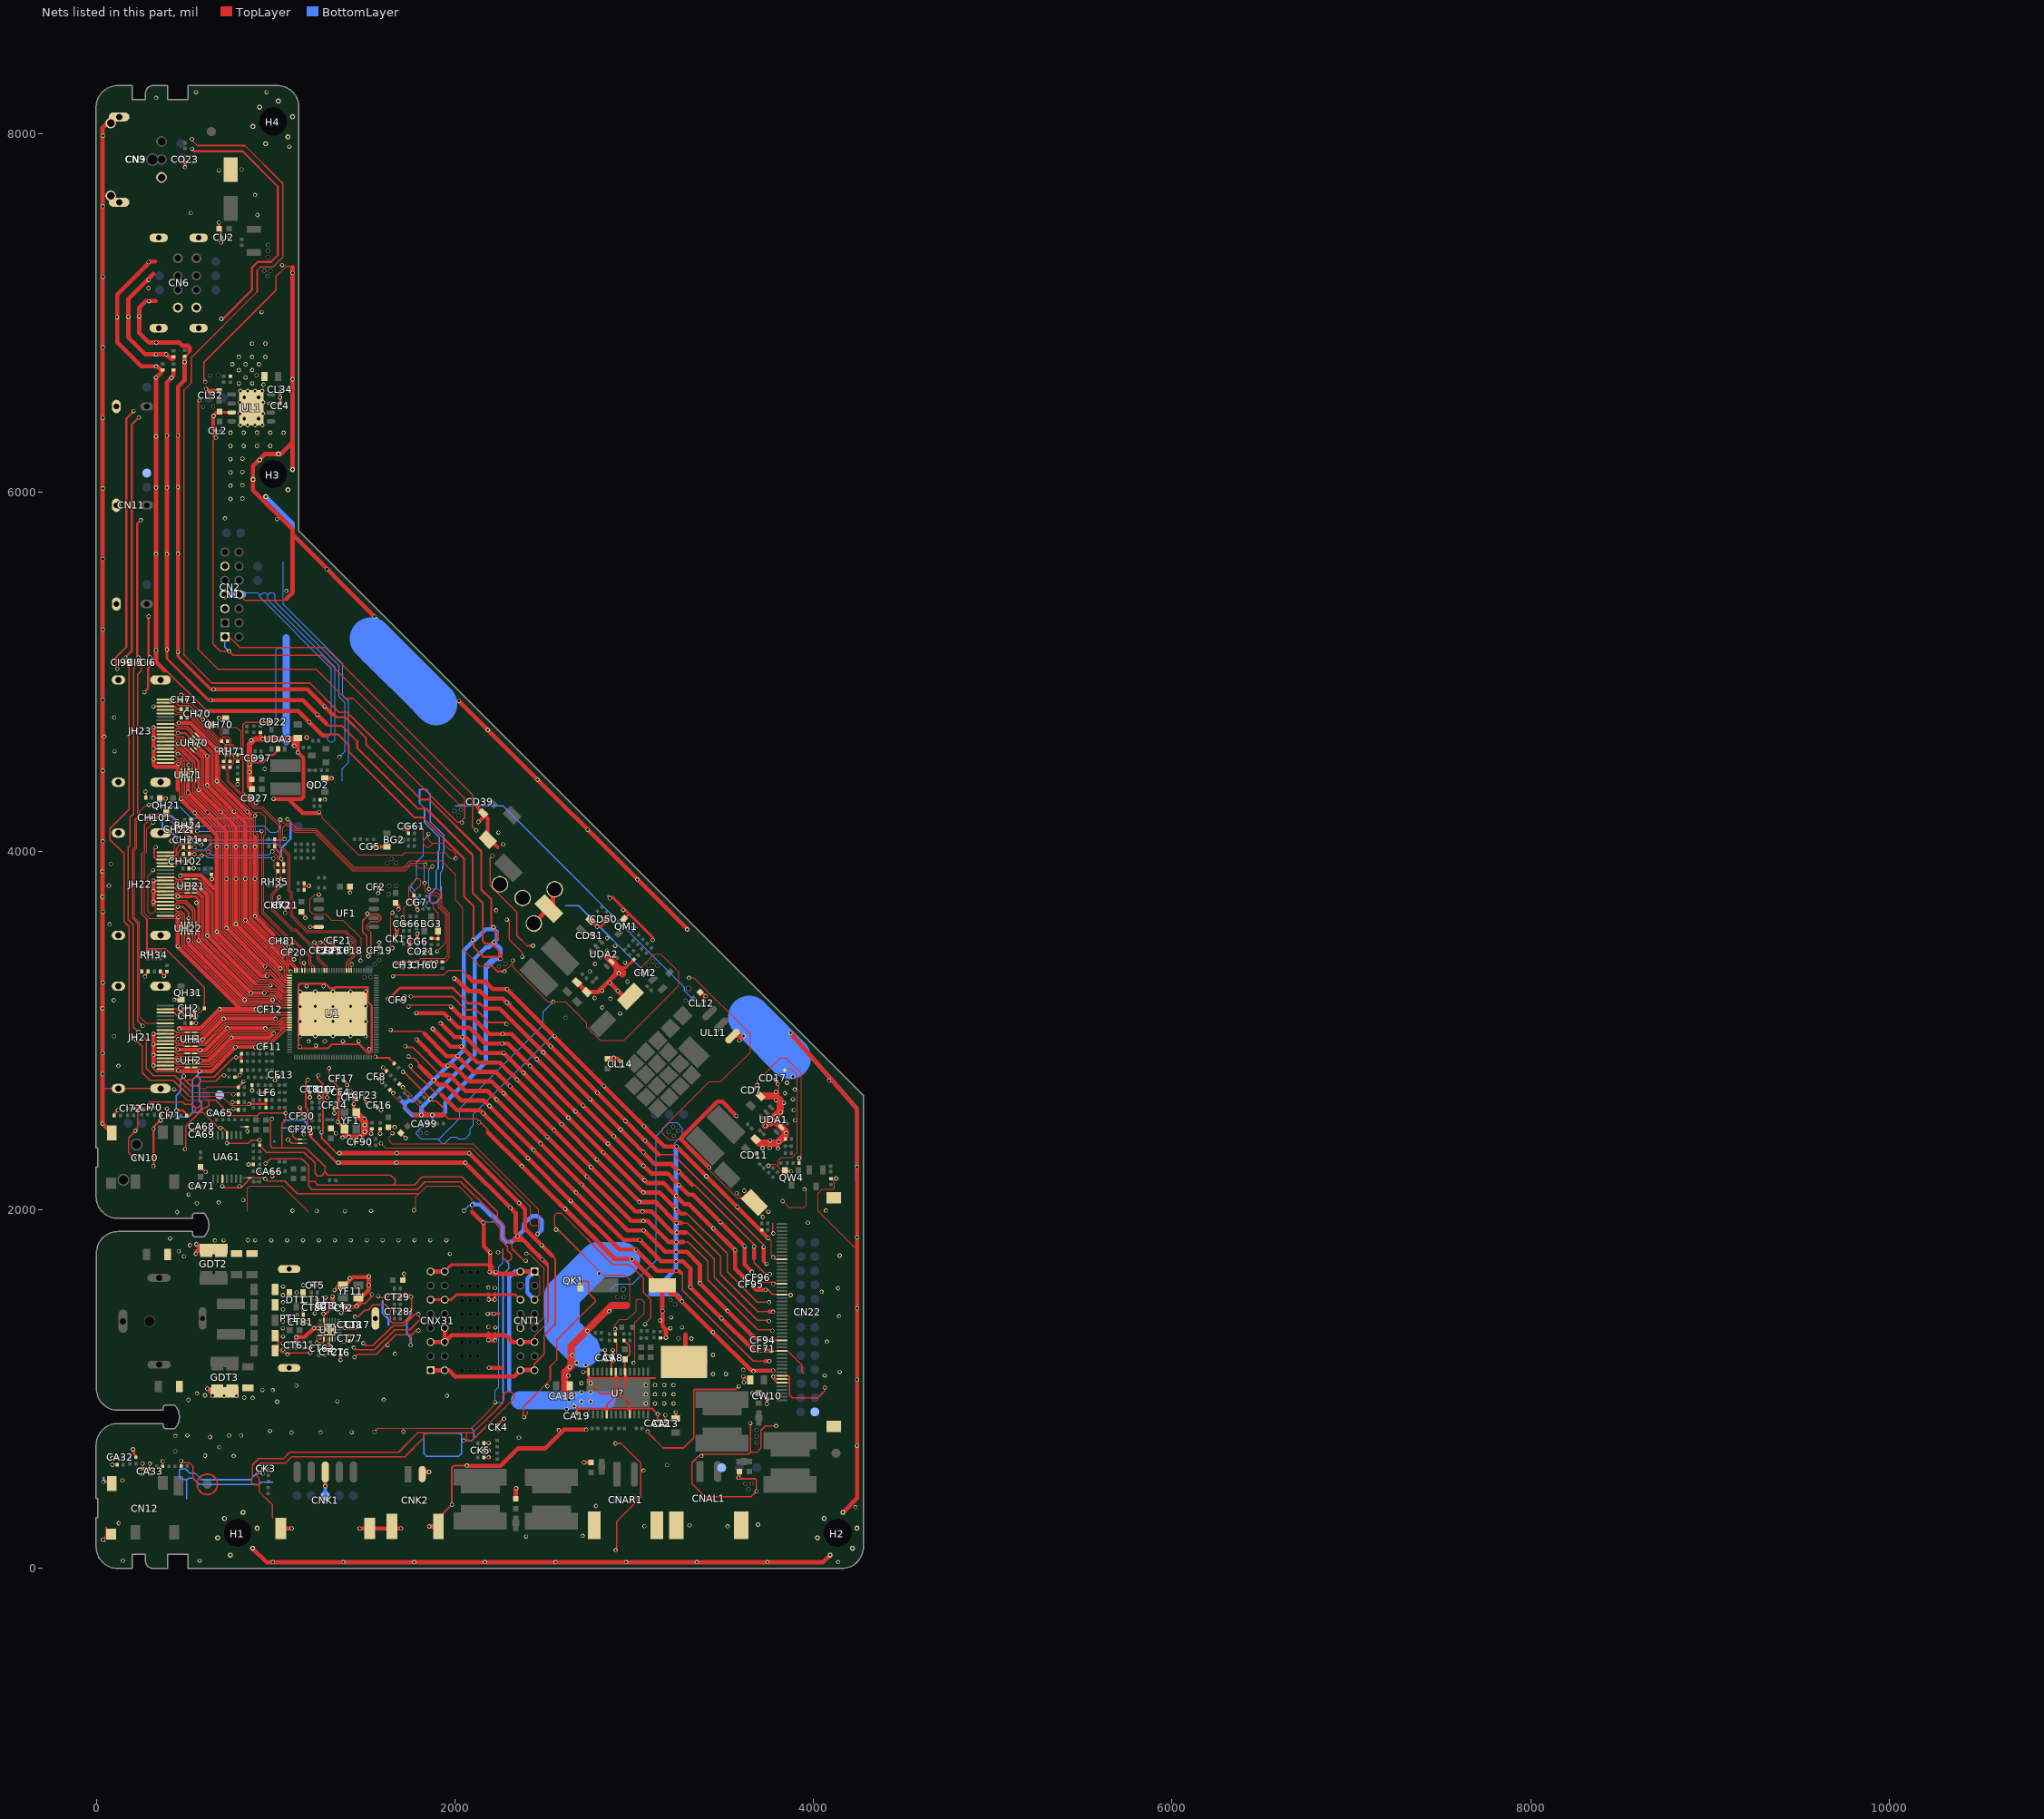
[diagram p0: the nets of this part, all layers, seen from the top]
# Altium PCB MISC105950.PcbDoc (part 10 of 15)
Units mil, origin at the board's own origin, x right, y up, seen from the top; angles counter-clockwise.
Board outline 4280.62 x 8272.76 mil, 2 copper layers (TopLayer, BottomLayer), stack 61.855 mil thick; 541 components, 268 nets, 2324 pads, 1157 vias.

## Via types
v1: diameter 23.62, hole 15.75, TopLayer to BottomLayer, tented both sides, 1087 vias
v2: diameter 23.62, hole 15.75, TopLayer to BottomLayer, 51 vias
v3: diameter 27.56, hole 19.68, TopLayer to BottomLayer, 15 vias
v4: diameter 31.5, hole 19.68, TopLayer to BottomLayer, tented both sides, 4 vias

## Nets (pads, with @x,y where several pads share a name; then routed paths per layer and width w, separated by ;. In a path a pad name is that pad's centre, name@x,y a point inside that pad or via, vN(x,y) a via of type N, cw(c..) or ccw(c..) an arc to the next point about the centre after c; other vN are vias at no path point) (continued)
GND: (continued)
  BottomLayer w15: v1(683,7506.5) v1@683.5,7506 ; v1(1790,3671) v1@1790.5,3671.5 ; v1(2182,1418) v1(2216,1418) ; 2221.5,1529.5 2221.5,1531.5 ; v1@2272.51,831.51 v1(2272.51,832.26) ; v1@2856.5,3742 2856.5,3750.5 ; v1@2893,1333.5 v1(2893.5,1333.5) ; v1@3394,3188.67 v1@3394,3193 ; v1(3739.5,915.5) v1@3740,915
  BottomLayer w20: v1@453.32,2893 v1(453.5,2893) ; GND_KEY.1@1275.9,404.78 v1(1275.9,457.78) ; v1(2615.04,2003.23) v1@2618.53,1999.75
  BottomLayer w24: v1@385,4293 v1(385.5,4292.5) ; v2(556,1806) v2@558,1808 ; H3.6@942.91,5977.37 1093.48,5826.8 1093.48,5711.6 ; 1563.52,5216.53 1563.52,5294.56 ; 1704.5,2600.5 1709.62,2600.5 1719.69,2590.43 ; 1817.55,2659.82 1818.62,2660.88 ; v1(1861.87,2615.5) v1@1859.5,2615.5 ; v1(2094.93,2025) 2104.24,2034.31 ; v1@2097.2,2026.9 2140.7,2026.9 2206.2,1961.4 2206.2,1971.8 2264,1914 2264,1841.81 2285.81,1820 ; 2170.95,3342.45 2225,3396.5 ; 2198,3388 2187,3377 ; v1@2219,1643.5 v1(2226.5,1651) ; 2223.69,1956.93 2223.81,1957.06 ; v1@2289,3155.5 2291.5,3155.5 2303,3144 ; 2300.5,1820 2318.28,1820 2383.5,1885.22 2383.5,1917.69 2428.62,1962.81 ; 2301.5,992.2 2301.5,1063.5 ; 2301.5,1030 2301.5,1063.5 ; CNT1.5@2443.21,1496.63 2403,1536.84 2403,1559.11 2403.12,1559.23 2403.12,1614.02 CNT1.1@2443.21,1654.11 2332.11,1654.11 2301.5,1623.5 2301.5,1063.5 ; 2445,1962.81 2428.62,1962.81 ; v1(2460,1863.5) 2483,1886.5 2483,1940 2460.19,1962.81 ; 2470.29,1952.71 2460.19,1962.81 ; 3034.5,2259.97 v1(3050.97,2243.5) ; 3041.25,2328.18 v1(3051.06,2318.37) ; v1(3235.87,2351.5) 3232,2347.63 3232,1669.51 3089.49,1527 3235.78,1527 3256,1506.78 ; 3861.04,2997.04 4243.09,2561.99 4243.09,2162 ; 1719.69,2590.43 1719.69,2566.57 1758.88,2527.38 1812.43,2527.38 v1(1812.5,2527.31) ; 1719.69,2590.43 1736.57,2607.31 1765.04,2607.31 1818.62,2660.88 ; v1(1812.5,2527.31) 1928.79,2527.31 1945.67,2544.19 1945.67,2595.95 2170.95,2821.23 2170.95,3360.95 2187,3377 ; v1(1812.5,2527.31) 1812.5,2568.5 v1@1859.5,2615.5 ; 1818.62,2660.88 2048.95,2891.21 2048.95,3443.56 2169.69,3564.31 2216.93,3564.31 2233.81,3547.43 2233.81,3508.81 v1(2216.5,3491.5) ; v1@1859.5,2615.5 2109.95,2865.95 2109.95,3400.45 2172.12,3462.62 2187.62,3462.62 v1(2216.5,3491.5) ; 2187,3377 2190.62,3377 2210.12,3396.5 2225,3396.5 ; v1(2216.5,3491.5) 2252.81,3455.19 2252.81,3398.31 2251,3396.5 2225,3396.5 ; 2428.62,1962.81 2460.19,1962.81
  BottomLayer w30: v1(1103,4588) v1@1104,4589
  BottomLayer w40: CN2.5@715.6,5431.32 CN2.6@815.18,5431.32 ; 1057.81,4611 1057.81,5188.69
  BottomLayer w100: 2360.5,935 2845.5,935
  BottomLayer w196.85: 2712.1,1215.9 2597.5,1330.5 2597.5,1522.47 2795.46,1720.43 2933,1720.43
  BottomLayer w236.22: 1530.5,5184.48 1530.5,5183.51 1580.96,5133.05 1581.92,5133.05 1859.43,4855.54 1859.43,4854.58 1894.08,4819.93 1895.04,4819.93 ; 3640.95,3074.03 3640.95,3073.1 3675.59,3038.46 3676.52,3038.46 3868.42,2846.56
  other v1: 983.5,32.5 1377.7,32.5 1771.9,32.5 2166.1,32.5 2560.3,32.5 2954.5,32.5 3348.7,32.5 3742.91,32.5 4137.11,32.5 2396,175.5 2711.5,179.5 3520.5,232.5 3056.5,233 3308,238 3690,242 4233,339 2786,345.5 3051.5,544 3182.7,575.1 4242,681.9 2356.2,726.9 1712,761 2578.5,769.1 1007,928 1342.5,930 1602,939 871,949 824,951 779,960 711,961 1954.5,961 647,962 605,963 560,974 983,992 925,993 4063,1006 3583,1013 2515,1014 1114.5,1018 4242.46,1050.7 4062,1074 4145.5,1094 3665,1098 3608,1106 1065.5,1191.68 1664.5,1194.5 1040,1217.5 1039,1253.5 4074.5,1262.5 2224,1270.5 3246,1281 1040,1291.5 1280.8,1311.3 1318.2,1311.3 1039,1337 2225,1342 3266,1342 2186,1344 1280.8,1348.7 1318.2,1348.7 1039,1376 3144,1381 3205,1398 4142.5,1404.5 1040,1443 4243.09,1449.2 1040,1483 1754,1514 1040,1522.5 1116.5,1536.5 4045,1541 1327,1550 4137,1561 2222,1562 2186,1564 1040,1570 1153,1578 2803.5,1643 488,1739 4145.5,1742.5 1971,1752 2239.5,1761.5 459,1767 520.5,1801 660,1827 707.8,1828 885.4,1828 974.2,1828 1063,1828 1151.8,1828 1240.6,1828 1329.4,1828 1418.2,1828 1507,1828 1595.8,1828 1684.6,1828 1773.4,1828 1862.2,1828 1951,1828 844,1829 4243.09,1844.2 3968.5,1926.5 1385.5,1990 1228,1992 1092.5,1993.5 4069,1994 818,2053 3233.92,2076.47 4243.09,2237.2 3801,2341 3715,2343 3756,2344 3805.06,2378.06 3757,2385 3846.16,2426.97 3759.63,2496.63 3897,2498 3786,2518 3817,2542 3889,2554 247.5,2567 3835,2595 3790,2610 3885,2615 3840,2649 904.5,2653 3790,2656 3895,2670 3852,2707 4086.26,2720.24 3884,2741 32.5,2756.5 122,2801.5 2887,2813 33.5,2873.01 1520.5,2895 1135.25,2908.25 1223,2914.5 1182.5,2938 1273,2938.5 1374,2939 1462,2939 97.5,2966.5 1135.43,2965.89 1501.57,2965.89 1318.97,2967.4 1220.07,2967.86 1416.93,2967.86 234,2990.5 2287.5,3035 1135.43,3048.57 1501.57,3048.57 1318.97,3050.07 1220.07,3050.54 1416.93,3050.54 1965.21,3068.35 2920.5,3093.5 1783.72,3095.81 32.5,3122 2821,3127 1135.43,3131.25 1220.07,3133.22 1318.97,3132.75 1416.93,3133.22 1501.57,3134.2 95.5,3167.5 2866.5,3176 2778,3180 1135.43,3213.92 1318.97,3215.43 1501.57,3215.43 1220.07,3215.89 1416.93,3215.89 2908.14,3219.36 2820,3220 1172,3245.5 1267,3246 2862.62,3264.88 34.5,3266.71 2962.5,3271 2913,3317.5 2751.5,3328.5 2780.5,3370 2949,3377 1101,3395 2811,3406.5 1900,3440.5 2849,3444.5 2892.5,3470.5 2848,3514.5 72.5,3591 512.98,3625 34.5,3660.41 2938,3670.5 557,3711.5 2863.5,3735.5 32.5,3744.5 581.95,3789.33 68.5,3806.5 3016.8,3841.28 724.5,3844.5 883.5,3844.5 32.5,3886.5 80,3928 537.23,3943.5 670.66,4023.5 724.5,4023.5 830.5,4023.5 883.5,4023.5 1573,4024 2267.6,4037.1 34.5,4054.12 2241.8,4103.1 2118,4115.5 2739.53,4118.56 2460.79,4397.3 34.5,4447.82 938,4458.3 512.98,4480 853.65,4483 100,4556.5 863.5,4618.1 1062.1,4624.5 963.2,4626.8 1014.5,4627.4 43.5,4638.86 2181.99,4676.09 1186,4718.5 98,4745.5 1231.5,4761.15 34.5,4841.52 653,4902.5 332,5120 34.5,5235.22 1058.86,5451 1284.78,5573.3 34.5,5628.92 332,5656 393,5656 454,5658.5 1006.04,5852.04 716,5856 34.5,6022.62 332,6313.5 393,6317 454,6317 802.58,6376.63 843.19,6376.63 883.81,6376.63 924.42,6376.63 34.5,6416.32 236.13,6418.51 798.42,6440.87 928.58,6440.87 206.8,6454.6 798.42,6503.13 928.58,6503.13 1023.5,6531 802.58,6567.37 843.19,6567.37 883.81,6567.37 924.42,6567.37 931,6602 1092.85,6632.5 418,6640 331,6642 892,6654 332,6703.76 491,6728 331,6770.76 34.5,6810.02 333,6836.26 696.5,6969 114.66,6978.5 177,6981 238,6983.5 920.5,7006 291.9,7067 290,7141 290.5,7186 34.5,7203.72 1035.5,7269 289.8,7286.7 897,7548 526,7560 34.5,7597.42 884,7660.5 682,7798 808.5,7802.5 1076,7930 34.5,7991.12 332.5,8202 554.5,8233.5 948.2,8233.5
  other v2: 147,41 574.5,41.5 123.5,249.5 144,489 764.5,625 605.5,627 439.5,651 685,673.5 633.5,730.5 439.5,736.5 739.5,739.5 805.5,739.5 506.5,740 1087,755.5 1249,756.5 1423,757.5 966.5,765 512.5,938 553.5,1752.5 410.5,1838 1531.5,1992.5 1770.5,1996 559.5,2035 681,2039.5 513,2083.5
  other v4: 824.13,6412.94 902.87,6412.94 824.13,6531.06 902.87,6531.06
GVDD: CA8.2@2881.84,1155.77 CA8.2@2881.84,1162.66 RA10.1 U?.9 | length 217.7
  TopLayer w10: U?.9@2871.82,1094.5 U?.9@2871.82,1113.5 ; 2871.82,1133.32 U?.9@2871.82,1113.5 ; RA10.1@2892.67,1263.5 2901.69,1254.48 2901.69,1236.5 ; 2901.69,1245 2901.69,1236.5 ; U?.9@2871.82,1113.5 2871.82,1145.75 CA8.2@2881.84,1155.77 2889.06,1155.77 2901.69,1168.4 2901.69,1236.5
HDMI_A_0N_IN_IC: JH23.9 U1.1 UH70.3 UH70.6 | length 1731.4
  TopLayer w7: JH23.9@384.16,4649.61 435.16,4649.61 449,4635.77 482.87,4635.77 500.12,4618.53 ; 500.12,4618.68 500.12,4618.53 ; 560.22,4558.42 560.22,4563.65 UH70.6@547.26,4576.61 UH70.3@518.3,4605.56 505.34,4618.53 500.12,4618.53 ; 561.28,4557.36 596.98,4521.66 596.98,4359.49 810,4146.48 810,3606.05 967.27,3448.77 ; 938.02,3478.02 967.27,3448.77 ; U1.1@1076.34,3305.46 1063.18,3305.46 1058,3310.64 1058,3358.05 967.27,3448.77
HDMI_A_0P_IN_IC: JH23.7 U1.2 UH70.4 UH70.5 | length 1761.3
  TopLayer w7: JH23.7@384.16,4610.24 432.97,4610.24 446.5,4623.77 ; 446.61,4623.66 478.01,4623.66 490.57,4611.1 490.57,4605.46 UH70.4@504.38,4591.64 UH70.5@533.34,4562.69 547.15,4548.88 552.8,4548.88 558.81,4542.87 584.98,4516.69 584.98,4354.52 798,4141.51 798,3601.08 1023.04,3376.04 ; 974.08,3425 1023.04,3376.04 ; U1.2@1076.34,3291.68 1059.99,3291.68 1046,3305.67 1046,3353.08 1023.04,3376.04
HDMI_A_1N_IN_IC: JH23.6 U1.3 UH71.1 UH71.8 | length 1656.7
  TopLayer w7: JH23.6@384.16,4590.55 435.16,4590.55 449,4576.72 470.66,4576.72 548.66,4498.71 548.66,4466.33 552.35,4462.64 UH71.1@552.35,4444.3 552.35,4385.02 548.66,4381.33 548.66,4332.87 757,4124.52 757,3584.09 1034,3307.09 1034,3300.23 1056.33,3277.9 U1.3@1076.34,3277.9
HDMI_A_1P_IN_IC: JH23.4 U1.4 UH71.2 UH71.7 | length 1666.6
  TopLayer w7: JH23.4@384.16,4551.18 432.97,4551.18 446.5,4564.72 465.68,4564.72 536.66,4493.74 536.66,4467.83 532.67,4463.84 532.67,4383.82 536.66,4379.83 536.66,4351 ; 536.66,4341.98 536.66,4351 ; U1.4@1076.34,3264.12 1053.14,3264.12 1022,3295.26 1022,3302.12 745,3579.12 745,4119.55 536.66,4327.9 536.66,4351
HDMI_A_2N_IN_IC: JH23.3 U1.5 UH71.3 UH71.6 | length 1647.4
  TopLayer w7: JH23.3@384.16,4531.5 435.16,4531.5 449,4517.66 470.56,4517.66 489.6,4498.62 489.6,4467.83 ; 489.6,4466.33 493.3,4462.64 493.3,4385.02 489.6,4381.33 489.6,4316.97 704,4102.57 704,3562.14 930.52,3335.62 964.67,3335.62 1049.95,3250.34 U1.5@1076.34,3250.34
HDMI_A_2P_IN_IC: JH23.1 U1.6 UH71.4 UH71.5 | length 1649.8
  TopLayer w7: JH23.1@384.16,4492.13 432.97,4492.13 446.5,4505.66 465.59,4505.66 477.6,4493.65 477.6,4467.83 473.61,4463.84 UH71.4@473.61,4444.3 473.61,4383.82 477.6,4379.83 477.6,4312 692,4097.6 692,3557.17 925.55,3323.62 959.7,3323.62 1046.76,3236.56 U1.6@1076.34,3236.56
HDMI_A_5V: CH70.1 JH23.18 RH70.2 RH71.2 RH71.4 RH71.6 RH74.2 | length 1006.3
  TopLayer w5: 744.5,4589.98 747.59,4593.07 747.59,4593.16 747.59,4624.95 733.2,4639.34 701.62,4639.34 692.81,4648.15 692.81,4685.85 697.21,4690.25 781.25,4690.25 805.15,4666.35 805.15,4597.42 805.15,4517.39 RH74.2@787.75,4499.99
  TopLayer w8: JH23.18@384.16,4826.77 443.23,4826.77 457.67,4812.33 517.82,4812.33 546,4784.15 546,4749.26 564.63,4730.63 ; 574.57,4720.69 564.63,4730.63 ; 651.88,4643.38 645.88,4649.38 ; RH70.2@697.3,4612 683.26,4612 645.88,4649.38 ; RH70.2@697.54,4611.77 716.15,4593.16 ; RH71.2@720.88,4573.5 720.88,4588.43 716.15,4593.16 ; 741.32,4593.16 716.15,4593.16 ; RH71.4@744.5,4573.5 744.5,4589.98 ; 744.5,4593.16 747.59,4593.16 757.84,4593.16 764.19,4586.81 RH71.6@764.19,4573.5 ; 564.63,4730.63 645.88,4649.38
HDMI_A_CKN_IN_IC: JH23.12 U1.127 UH70.1 UH70.8 | length 1746.2
  TopLayer w7: JH23.12@384.16,4708.66 435.16,4708.66 449,4694.83 507.34,4694.83 541.88,4660.29 ; 541.88,4660.44 541.88,4660.29 ; U1.127@1118.7,3334.04 1118.7,3348.26 1074.21,3392.75 1074.21,3416.79 863,3628 863,4168.43 649.98,4381.45 649.98,4552.18 601.98,4600.18 601.98,4605.41 UH70.8@589.01,4618.37 UH70.1@560.06,4647.32 547.1,4660.29 541.88,4660.29
HDMI_A_CKP_IN_IC: JH23.10 U1.128 UH70.2 UH70.7 | length 1725.5
  TopLayer w7: JH23.10@384.16,4669.29 432.97,4669.29 446.5,4682.83 446.61,4682.72 502.47,4682.72 532.33,4652.86 532.33,4647.22 UH70.2@546.14,4633.4 UH70.7@575.1,4604.45 588.91,4590.64 594.56,4590.64 637.98,4547.21 637.98,4376.48 851,4163.46 851,3623.03 1062.21,3411.82 1062.21,3387.78 1104.92,3345.07 U1.128@1104.92,3334.04
HDMI_A_HPD_OUT: CH71.1 JH23.19 QH70.C RH70.1 | length 476.1
  TopLayer w5: JH23.19@384.16,4846.46 CH71.1@468.81,4846.46 ; CH71.1@471.77,4840.23 471.77,4828.73 475.67,4824.83 529.98,4824.83 623.65,4731.15 623.65,4718.16 636.81,4705 QH70.C@641.97,4705 641.97,4669.55 682.18,4629.34 713.89,4629.34 RH70.1@731.23,4612 ; CH71.1@471.77,4843.5 CH71.1@473.4,4841.86
HDMI_A_HPD_OUT_IC: RH71.5 RH71.7 U1.120 | length 1571.8
  TopLayer w5: RH71.5@764.19,4538.07 766.5,4535.75 766.5,4516.5 ; RH71.7@787.81,4538.07 787.81,4520.81 783.5,4516.5 766.5,4516.5 ; U1.120@1215.15,3334.04 1215.15,3353.63 1195.66,3373.13 1195.66,3411.08 1090.27,3516.47 1073.53,3516.47 933,3656.99 933,4086 941.81,4094.81 941.81,4187.66 912.48,4216.98 871.02,4216.98 689.98,4398.01 689.98,4477.06 695.55,4482.63 756.7,4482.63 766.5,4492.42 766.5,4516.5
HDMI_A_SCL_IN: DH71.K JH23.15 RH71.1 RH72.1 | length 491.3
  TopLayer w5: JH23.15@384.16,4767.72 432.78,4767.72 437.67,4762.83 487.9,4762.83 DH71.K@506.23,4744.5 520.35,4744.5 693.54,4571.31 693.54,4543.96 699.43,4538.07 RH71.1@720.88,4538.07 720.88,4512.11 RH72.1@708.5,4499.73
HDMI_A_SCL_IN_IC: RH72.2 U1.107 | length 1616.3
  TopLayer w5: RH72.2@708.5,4466.27 708.5,4466 728.81,4445.69 728.81,4387.47 779.42,4336.86 ; 767,4349.28 779.42,4336.86 ; U1.107@1394.29,3334.04 1394.19,3334.13 1394.19,3381.25 1435.31,3422.37 1435.31,3496 1385,3546.31 1173.56,3546.31 1121.24,3598.64 1121.02,3598.64 1081,3638.66 1081,3766 1070.36,3776.64 1070.36,3974.64 1019.86,4025.14 1019.86,4138.1 933.96,4224 933.75,4224 920.77,4236.98 879.3,4236.98 779.42,4336.86
HDMI_A_SDA_IO: DH72.K JH23.16 RH71.3 RH73.1 | length 527.9
  TopLayer w5: JH23.16@384.16,4787.4 433.6,4787.4 448.17,4772.83 487.56,4772.83 DH72.K@506.23,4791.5 527.42,4770.31 527.42,4751.57 703.54,4575.46 703.54,4560.55 708.68,4555.41 733.83,4555.41 RH71.3@744.5,4544.74 ; RH73.1@744.5,4506.23 RH71.3@744.5,4538.07
HDMI_A_SDA_IO_IC: RH73.2 U1.106 | length 1608.4
  TopLayer w5: 738.81,4392.7 738.81,4391.61 ; RH73.2@744.5,4466.27 738.81,4460.58 738.81,4391.61 ; 1257.5,3556.31 1265.5,3556.31 ; U1.106@1406.12,3329 U1.106@1406.12,3334.04 ; U1.106@1408.07,3334.04 1408.07,3356.52 1404.19,3360.39 1404.19,3377.11 1445.31,3418.23 1445.31,3500.14 1389.14,3556.31 1265.5,3556.31 ; 738.81,4391.61 883.44,4246.98 924.91,4246.98 937.89,4234 938.1,4234 1029.86,4142.24 1029.86,4029.28 1080.36,3978.78 1080.36,3780.78 1091,3770.14 1091,3642.8 1125.16,3608.64 1125.38,3608.64 1177.7,3556.31 1265.5,3556.31
HDMI_ARC_OUT: CH81.1 DH81.K JH21.14 | length 2780.3
  TopLayer w5: v1@287,4253 272.31,4253 240.31,4221 240.31,4182 225,4166.69 225,4016.26 211.5,4002.76 211.5,3630.31 239.5,3602.31 239.5,3341.77 DH81.K@252.77,3328.5 239.5,3315.23 239.5,3074.5 274.63,3039.37 JH21.14@384.16,3039.37 ; v1@886,4195.5 886,4104.08 903,4087.08 903,3644.57 1025.17,3522.4 CH81.1@1025.17,3508.83
  BottomLayer w5: v1(291.5,4257.5) 300.81,4266.81 339.5,4266.81 359.95,4246.36 465.09,4246.36 526.95,4184.5 871,4184.5 v1(884,4197.5)
HDMI_ARC_OUT_IC: CH81.2@1043.96,3490.04 CH81.2@1048.83,3485.17 U1.125 | length 210.2
  TopLayer w5: CH81.2@1048.83,3485.17 1049.98,3486.31 1078,3486.31 1137.31,3427 1137.31,3369.24 1146.26,3360.3 U1.125@1146.26,3334.04
HDMI_B_0N_IN_IC: JH22.9 U1.9 UH21.3 UH21.6 | length 1076.2
  TopLayer w7: JH22.9@384.16,3795.28 435.16,3795.28 449,3781.44 484.39,3781.44 484.5,3781.33 488.19,3785.02 UH21.3@506.53,3785.02 UH21.6@547.47,3785.02 557.27,3785.02 597.16,3745.13 597.16,3519.08 874.42,3241.81 950.12,3241.81 961.93,3230 1002.41,3230 1037.19,3195.22 U1.9@1076.34,3195.22
HDMI_B_0P_IN_IC: JH22.7 U1.10 UH21.4 UH21.5 | length 1073.6
  TopLayer w7: JH22.7@384.16,3755.91 432.97,3755.91 446.5,3769.44 ; 446.61,3769.33 483,3769.33 486.99,3765.34 UH21.4@506.53,3765.34 UH21.5@547.47,3765.34 559.98,3765.34 585.16,3740.16 585.16,3514.11 869.45,3229.81 945.15,3229.81 956.96,3218 997.44,3218 1034,3181.44 U1.10@1076.34,3181.44
HDMI_B_1N_IN_IC: JH22.6 U1.11 UH22.1 UH22.8 | length 1082.8
  TopLayer w7: JH22.6@384.16,3736.22 435.16,3736.22 449,3722.39 ; 484.5,3722.39 449,3722.39 ; U1.11@1076.34,3167.66 1030.81,3167.66 995.47,3203 969.46,3203 955.46,3189 852.28,3189 838.28,3203 548.66,3492.62 548.66,3527 552.35,3530.69 UH22.8@552.35,3549.03 UH22.1@552.35,3589.97 552.35,3608.31 548.66,3612 548.66,3671.84 498.11,3722.39 449,3722.39
HDMI_B_1P_IN_IC: JH22.4 U1.12 UH22.2 UH22.7 | length 1094.6
  TopLayer w7: JH22.4@384.16,3696.85 432.97,3696.85 446.5,3710.39 466,3710.39 ; 483,3710.39 466,3710.39 ; 648.5,3375.81 669.3,3355.02 ; U1.12@1076.34,3153.89 1027.61,3153.89 990.5,3191 974.43,3191 960.43,3177 847.31,3177 669.3,3355.02 ; 466,3710.39 493.14,3710.39 536.66,3666.87 536.66,3613.5 532.67,3609.51 UH22.2@532.67,3589.97 UH22.7@532.67,3549.03 532.67,3529.49 536.66,3525.5 536.66,3487.65 669.3,3355.02
HDMI_B_2N_IN_IC: JH22.3 U1.13 UH22.3 UH22.6 | length 1053.4
  TopLayer w7: JH22.3@384.16,3677.17 435.16,3677.17 449,3663.33 472.47,3663.33 489.6,3646.2 489.6,3613.5 ; 489.6,3612 493.3,3608.31 UH22.3@493.3,3589.97 UH22.6@493.3,3549.03 493.3,3530.69 489.6,3527 489.6,3476.73 633.29,3333.04 ; 607.5,3358.83 633.29,3333.04 ; U1.13@1076.34,3140.11 1056.28,3140.11 1054.5,3138.33 1018.77,3138.33 1007.1,3150 816.33,3150 633.29,3333.04
HDMI_B_2P_IN_IC: JH22.1 U1.14 UH22.4 UH22.5 | length 1046.2
  TopLayer w7: JH22.1@384.16,3637.8 432.97,3637.8 446.5,3651.33 467.5,3651.33 477.6,3641.23 477.6,3613.5 473.61,3609.51 UH22.4@473.61,3589.97 UH22.5@473.61,3549.03 473.61,3529.49 477.6,3525.5 477.6,3471.75 615.56,3333.79 ; 595.5,3353.86 615.56,3333.79 ; U1.14@1076.34,3126.33 1013.8,3126.33 1002.13,3138 811.36,3138 615.56,3333.79
HDMI_B_5V: CH21.1 JH22.18 RH1.2 RH23.2 RH24.2 RH24.4 RH24.6 | length 2572.1
  TopLayer w5: v1(1049.17,4066.69) 1039.86,4076 1039.86,4131.81 1051.17,4143.12 1067.17,4143.12 1104.79,4105.5 1213.28,4105.5 1427.78,3891 1722.49,3891 1751.3,3919.81 1782.9,3919.81 1797.03,3905.69 v1@1873.19,3905.69 ; v1(1854.5,3788) 1905.5,3788 1926.5,3767 1926.5,3694.14 1968.31,3652.33 1968.31,3404.54 1944.5,3380.73 RH1.2@1929,3380.73
  TopLayer w8: JH22.18@384.16,3972.44 440.18,3972.44 445.74,3978.01 445.74,4014.93 473.37,4042.55 512.55,4042.55 517.07,4047.07 CH21.1@517.07,4056.98 ; 470.84,4132.5 RH24.4@491.5,4132.5 ; 491.5,4097.34 CH21.1@517.07,4071.77 ; RH24.2@491.5,4108.88 472.12,4108.88 468.34,4112.66 468.34,4146.34 474.19,4152.18 RH24.6@491.5,4152.18 ; CH21.1@517.07,4067.93 CH21.1@517.07,4062.1 517.68,4061.5 v1(543.74,4061.5) RH23.2@573.77,4061.5
  BottomLayer w5: v1(543.74,4061.5) v1@1043.98,4061.5 ; v1(1854.5,3788) 1854.5,3894.5 v1(1874,3914)
HDMI_B_CKN_IN_IC: JH22.12 U1.7 UH21.1 UH21.8 | length 1089.3
  TopLayer w7: JH22.12@384.16,3854.33 435.16,3854.33 449,3840.5 484.39,3840.5 484.5,3840.39 488.19,3844.08 UH21.1@506.53,3844.08 UH21.8@547.47,3844.08 565.81,3844.08 573.49,3836.39 580.85,3836.39 650.16,3767.09 650.16,3541.03 908.57,3282.62 983.73,3282.62 1043.57,3222.78 U1.7@1076.34,3222.78
HDMI_B_CKP_IN_IC: JH22.10 U1.8 UH21.2 UH21.7 | length 1086.8
  TopLayer w7: JH22.10@384.16,3814.96 432.97,3814.96 446.5,3828.5 446.61,3828.39 483,3828.39 486.99,3824.39 UH21.2@506.53,3824.39 UH21.7@547.47,3824.39 575.88,3824.39 638.16,3762.12 638.16,3536.06 903.6,3270.62 978.76,3270.62 1040.38,3209 U1.8@1076.34,3209
HDMI_B_HPD_OUT: CH22.1 JH22.19 QH21.C RH23.1 | length 573.8
  TopLayer w5: JH22.19@384.16,3992.13 426.87,3992.13 434.24,3999.5 434.24,4010.5 ; QH21.C@388.5,4214.47 430.19,4172.78 430.19,4120.31 CH22.1@445.73,4104.77 ; v1(417,4056) 430.74,4056 ; 434.24,4035 434.24,4010.5 ; 434.24,4040.74 434.24,4056 ; CH22.1@449.5,4104.77 434.24,4089.51 434.24,4056 ; v1(585.23,4033.85) 579.58,4033.85 RH23.1@607.23,4061.5 ; 434.24,4010.5 434.24,4056
  BottomLayer w5: v1(417,4056) 431.95,4041.05 567.05,4041.05 574.26,4033.85 v1(585.23,4033.85)
HDMI_B_HPD_OUT_IC: RH24.5 RH24.7 U1.121 | length 1432.1
  TopLayer w5: RH24.5@526.93,4152.18 542.96,4152.18 ; RH24.7@526.93,4175.81 538.69,4175.81 544.28,4170.22 544.28,4130.72 v1@561,4114 ; v1@918.12,4110.88 v1(920.65,4110.88) 923,4108.53 923,3938 ; 923,4006.5 923,3938 ; U1.121@1201.37,3334.04 1201.37,3353.27 1186.66,3367.99 1186.66,3405.94 1086.28,3506.31 1069.54,3506.31 923,3652.85 923,3938
  BottomLayer w5: v1@561.38,4110.88 v1(920.65,4110.88)
  other v1: 561,4110.5
HDMI_B_SCL_IN: DH22.K DH75.K JH22.15 RH24.1 RH35.3 | length 1060.9
  TopLayer w5: JH22.15@384.16,3913.39 439.24,3913.39 453.5,3927.64 453.5,3952.27 DH22.K@485.33,3984.1 506.62,3962.81 557.5,3962.81 569.69,3975 v1(585.23,3975) ; RH24.1@526.93,4108.88 545,4090.81 628.08,4090.81 641.16,4077.73 641.16,3988.16 630.19,3977.19 592.64,3977.19 v1@585.23,3969.77 ; v1@991.81,3953 991.81,3906.23 DH75.K@1010.54,3887.5 1003.84,3880.81 RH35.3@1003.84,3844.22
  BottomLayer w5: v1@585.23,3969.77 v1@586.5,3971.05 ; v1@586.5,3974 607.81,3974 619.5,3962.31 v1@982.5,3962.31
  other v1: 986.07,3958.74
HDMI_B_SCL_IN_IC: RH35.4 U1.116 | length 620.5
  TopLayer w5: RH35.4@1003.84,3808.78 1003.84,3788.94 973,3758.09 973,3673.56 1090.1,3556.47 1106.84,3556.47 1231.66,3431.65 1231.66,3393.7 1270.27,3355.08 U1.116@1270.27,3334.04
HDMI_B_SDA_IO: DH23.K DH76.K JH22.16 RH24.3 RH35.1 | length 1107.4
  TopLayer w5: JH22.16@384.16,3933.07 438.57,3933.07 442.46,3936.96 442.46,3957.72 457.24,3972.5 457.24,3994.01 483.11,4019.89 500.57,4002.43 v1@615.57,4002.43 ; RH24.3@526.93,4132.5 520.26,4132.5 509.59,4121.83 509.59,4095.52 524.29,4080.81 623.93,4080.81 631.16,4073.59 631.16,4006.16 v1(621.5,3996.5) ; v1(981,3998.5) 1010.54,3968.96 DH76.K@1010.54,3926 1027.46,3909.07 RH35.1@1027.46,3844.22
  BottomLayer w5: v1(621.5,3996.5) 638.81,3979.19 961.69,3979.19 v1(981,3998.5)
HDMI_B_SDA_IO_IC: RH35.2 U1.115 | length 627.7
  TopLayer w5: RH35.2@1027.46,3808.78 1027.46,3798.42 983,3753.95 983,3677.71 1094.24,3566.47 1110.98,3566.47 1240.66,3436.79 1240.66,3398.84 1284.05,3355.44 U1.115@1284.05,3334.04
HDMI_C_0N_IN_IC: JH21.9 U1.18 UH1.3 UH1.6 | length 760.8
  TopLayer w7: JH21.9@384.16,2940.95 435.16,2940.95 449,2927.11 484.39,2927.11 484.5,2927 488.19,2930.69 UH1.3@506.53,2930.69 UH1.6@547.47,2930.69 565.81,2930.69 569.5,2927 599.94,2927 716.94,3044 1010.12,3044 1035.55,3069.43 1060.75,3069.43 1062.53,3071.21 U1.18@1076.34,3071.21
HDMI_C_0P_IN_IC: JH21.7 U1.19 UH1.4 UH1.5 | length 760
  TopLayer w7: JH21.7@384.16,2901.58 432.97,2901.58 446.5,2915.11 ; 446.61,2915 483,2915 486.99,2911.01 UH1.4@506.53,2911.01 UH1.5@547.47,2911.01 567.01,2911.01 571,2915 604.92,2915 721.92,3032 1015.09,3032 1040.52,3057.43 U1.19@1076.34,3057.43
HDMI_C_1N_IN_IC: JH21.6 U1.20 UH2.1 UH2.8 | length 784.3
  TopLayer w7: JH21.6@384.16,2881.89 435.16,2881.89 449,2868.06 484.5,2868.06 488.19,2871.75 UH2.1@506.53,2871.75 UH2.8@547.47,2871.75 565.81,2871.75 569.5,2868.06 615.95,2868.06 738.9,2991 950.05,2991 966.02,3006.98 ; 973.53,3014.49 966.02,3006.98 ; U1.20@1076.34,3043.65 1059.65,3043.65 1057.87,3041.87 1041.93,3041.87 1016.06,3016 975.05,3016 966.02,3006.98
HDMI_C_1P_IN_IC: JH21.4 U1.21 UH2.2 UH2.7 | length 773.1
  TopLayer w7: JH21.4@384.16,2842.52 432.97,2842.52 446.5,2856.06 483,2856.06 486.99,2852.06 UH2.2@506.53,2852.06 UH2.7@547.47,2852.06 567.01,2852.06 571,2856.06 620.92,2856.06 743.87,2979 955.02,2979 980.02,3004 1021.03,3004 1046.9,3029.87 U1.21@1076.34,3029.87
HDMI_C_2N_IN_IC: JH21.3 U1.22 UH2.3 UH2.6 | length 786.8
  TopLayer w7: JH21.3@384.16,2822.84 435.16,2822.84 449,2809 484.5,2809 488.19,2812.69 UH2.3@506.53,2812.69 UH2.6@547.47,2812.69 565.81,2812.69 569.5,2809 631.85,2809 760.85,2938 972,2938 1050.09,3016.09 U1.22@1076.34,3016.09
HDMI_C_2P_IN_IC: JH21.1 U1.23 UH2.4 UH2.5 | length 786.1
  TopLayer w7: JH21.1@384.16,2783.47 432.97,2783.47 446.5,2797 483,2797 486.99,2793.01 UH2.4@506.53,2793.01 UH2.5@547.47,2793.01 567.01,2793.01 571,2797 636.82,2797 765.82,2926 976.97,2926 1053.28,3002.31 U1.23@1076.34,3002.31
HDMI_C_5V: CH1.1 JH21.18 RH33.2 RH34.3 RH34.5 RH34.7 RH81.2 | length 4161.6
  TopLayer w5: v1(1025,4175) 1046.88,4153.12 1071.31,4153.12 1108.93,4115.5 1217.5,4115.5 1432,3901 1718.35,3901 1751.66,3934.31 1824.5,3934.31 v1(1833.81,3925) ; RH81.2@1786,3382.23 1793.43,3382.23 1811.7,3400.5 1945,3400.5 1958.31,3413.81 1958.31,3648.19 1916.5,3690 1916.5,3753 1901,3768.5 1842.5,3768.5 1832,3779 v1@1832,3819
  TopLayer w8: 281.84,3455.34 384.66,3455.34 600.23,3239.77 RH33.2@600.23,3123 577.07,3099.84 507.34,3099.84 495.77,3088.27 CH1.1@495.77,3081 481.93,3081 444.82,3118.11 JH21.18@384.16,3118.11 ; RH34.7@289.57,3436.5 281,3445.07 281,3619.5 253,3647.5 253,3985.57 268,4000.57 268,4149 281.81,4162.81 281.81,4192.22 295.93,4206.34 349.38,4206.34 357.25,4198.48 357.25,4193.91 v1@382.15,4169 ; RH34.5@310.69,3436.5 310.69,3452.04 ; RH34.3@330.38,3436.5 330.38,3453.72
  BottomLayer w5: v1(388.77,4173.43) 406.18,4173.43 439.42,4140.19 932.79,4140.19 968.79,4104.19 1004.19,4104.19 1025,4125 v1(1025,4175) ; v1(1829.5,3821.5) v1@1829.5,3925
HDMI_C_CKN_IN_IC: JH21.12 U1.16 UH1.1 UH1.8 | length 747.7
  TopLayer w7: JH21.12@384.16,3000 435.16,3000 449,2986.17 484.39,2986.17 484.5,2986.06 488.19,2989.75 UH1.1@506.53,2989.75 UH1.8@547.47,2989.75 565.81,2989.75 569.5,2986.06 584.05,2986.06 694.99,3097 1023.99,3097 1059.5,3096.99 1061.28,3098.77 U1.16@1076.34,3098.77
HDMI_C_CKP_IN_IC: JH21.10 U1.17 UH1.2 UH1.7 | length 766.1
  TopLayer w7: JH21.10@384.16,2960.63 432.97,2960.63 446.5,2974.17 446.61,2974.06 483,2974.06 486.99,2970.06 UH1.2@506.53,2970.06 UH1.7@547.47,2970.06 567.01,2970.06 571,2974.06 589.02,2974.06 699.96,3085 977.5,3085 ; 958.5,3085 977.5,3085 ; 1006.88,3085 977.5,3085 ; 1006.89,3084.99 U1.17@1076.34,3084.99